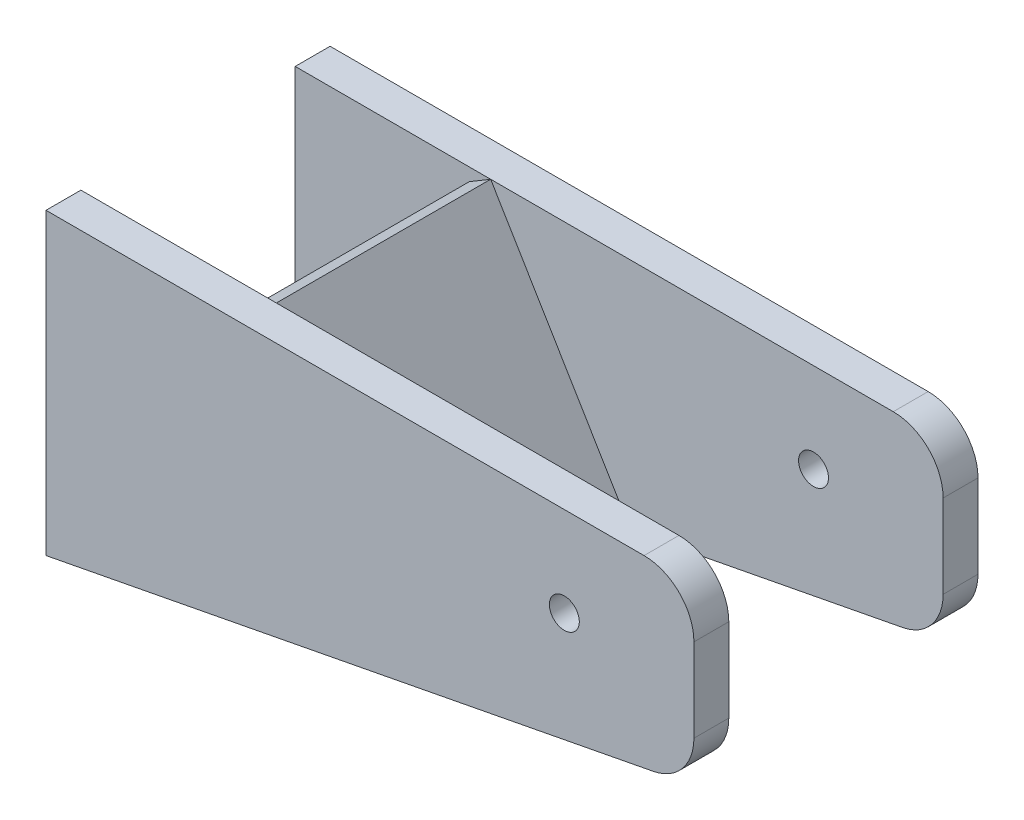
SolidWorks part; units mm, degrees
material "Q235铸造"
ref_plane "前视基准面" through (0, 0, 0) normal (0, 0, 1) x (1, 0, 0)
ref_plane "上视基准面" through (0, 0, 0) normal (0, 1, 0) x (1, 0, 0)
ref_plane "右视基准面" through (0, 0, 0) normal (1, 0, 0) x (0, 0, -1)
ref_plane "基准面1" through (686, 0, 0) normal (1, 0, 0) x (0, 0, -1)
sketch "草图1" plane through (686, 0, 0) normal (1, 0, 0) x (0, 0, -1)
  line L1 (1688, 122) -> (1695, 122)
  line L2 (1688, 122) -> (1688, 62)
  line L3 (1688, 62) -> (1695, 62)
  line L4 (1695, 122) -> (1695, 62)
  line L5 (2265, 129) -> (0, 129) construction
  dimension "D1" = 7
  dimension "D2" = 60
  dimension "D4" = 7
extrude "凸台-拉伸1" add sketch "草图1" along normal blind 130
sketch "草图2" plane through (0, 0, -1695) normal (0, 0, -1) x (-1, 0, 0)
  line L0 (-816, 87) -> (-686, 62)
  line L1 (-816, 62) -> (-816, 122) construction
  line L3 (-686, 38.5) -> (-686, -38.5) construction
  line L4 (-816, 62) -> (-686, 62) construction
  line L5 (-816, 87) -> (-816, 62)
  line L6 (-816, 62) -> (-686, 62)
  line L7 (-816, 122) -> (-686, 122) construction
  circle A0 centre (-790, 104) radius 3
  dimension "D2" = 6
  dimension "D3" = 18
  dimension "D4" = 26
  dimension "D1" = 35
extrude "切除-拉伸1" cut sketch "草图2" against normal through all
fillet "圆角1" radius 10 2 edges at (816, 122, -1691.5) (816, 87, -1691.5)
pattern_linear "阵列(线性)2" count 2 spacing 50 along (0, 0, 1) of bodies 107
sketch "草图3" plane through (0, 0, -1688) normal (0, 0, 1) x (1, 0, 0)
  line L0 (720.9289, 119.4334) -> (748.1351, 73.9491)
  line L2 (806, 122) -> (686, 122) construction
  line L3 (686, 62) -> (807.8885, 85.4401) construction
  line L4 (748.1351, 73.9491) -> (752.4261, 76.5157)
  line L5 (752.4261, 76.5157) -> (725.2199, 122)
  line L6 (725.2199, 122) -> (720.9289, 119.4334)
  dimension "D1" = 5
  dimension "D2" = 53
  dimension "D3" = 70
extrude "凸台-拉伸2" add sketch "草图3" along normal up to next separate body
ref_plane "基准面2" through (0, 103.6301, 0) normal (0, 1, 0) x (1, 0, 0)
ref_plane "基准面3" through (0, 0, -1666.5) normal (0, 0, 1) x (1, 0, 0)
